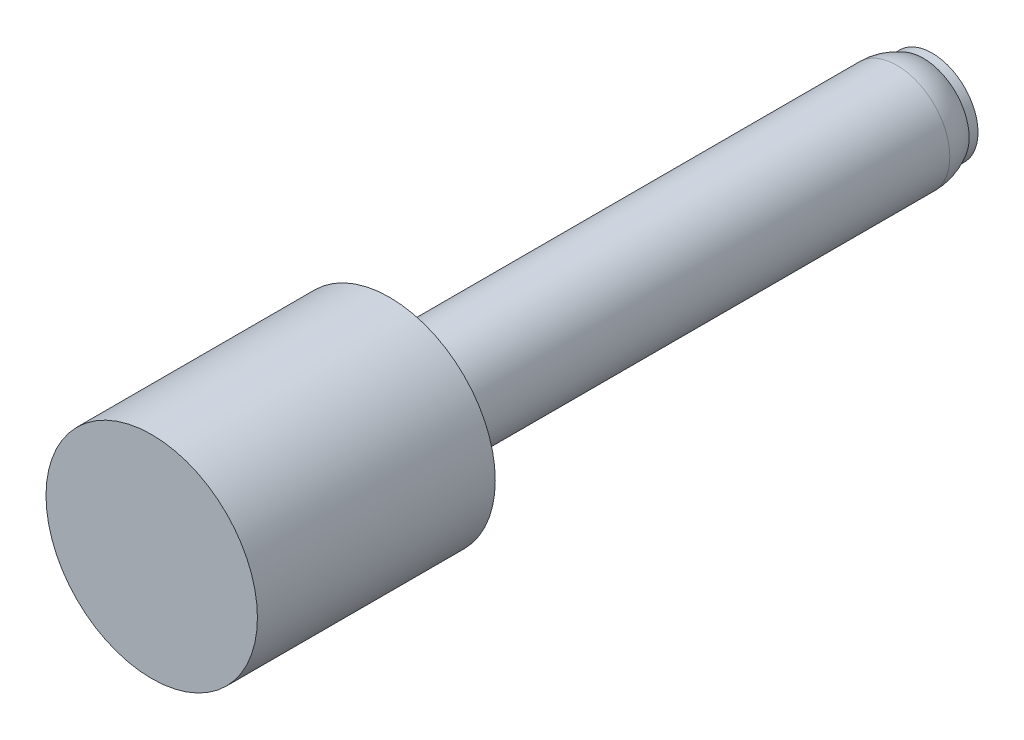
SolidWorks part; units mm, degrees
ref_plane "Front Plane" through (0, 0, 0) normal (0, 0, 1) x (1, 0, 0)
ref_plane "Top Plane" through (0, 0, 0) normal (0, 1, 0) x (1, 0, 0)
ref_plane "Right Plane" through (0, 0, 0) normal (1, 0, 0) x (0, 0, -1)
other "Configuration Table"
sketch "Sketch1" plane through (0, 0, 0) normal (0, 0, 1) x (1, 0, 0)
  circle A0 centre (599.8842, 0) radius 60
  dimension "D1" = 120
extrude "Boss-Extrude1" add sketch "Sketch1" against normal blind 135
sketch "Sketch2" plane through (0, 0, -135) normal (0, 0, -1) x (-1, 0, 0)
  circle A0 centre (-599.8842, 0) radius 30
extrude "Boss-Extrude2" add sketch "Sketch2" along normal blind 318 contours A0
fillet "Fillet2" radius 30 1 edges at (569.8842, 0, -453)
ref_plane "Plane1" through (0, 0, -423) normal (0, 0, 1) x (1, 0, 0)
sketch "Sketch3" plane through (0, 0, -423) normal (0, 0, 1) x (1, 0, 0)
  circle A0 centre (599.8842, 0) radius 30
  circle A1 centre (599.8842, 0) radius 26
  dimension "D1" = 60
  dimension "D2" = 4
extrude "Boss-Extrude3" add sketch "Sketch3" against normal blind 20 contours A1
